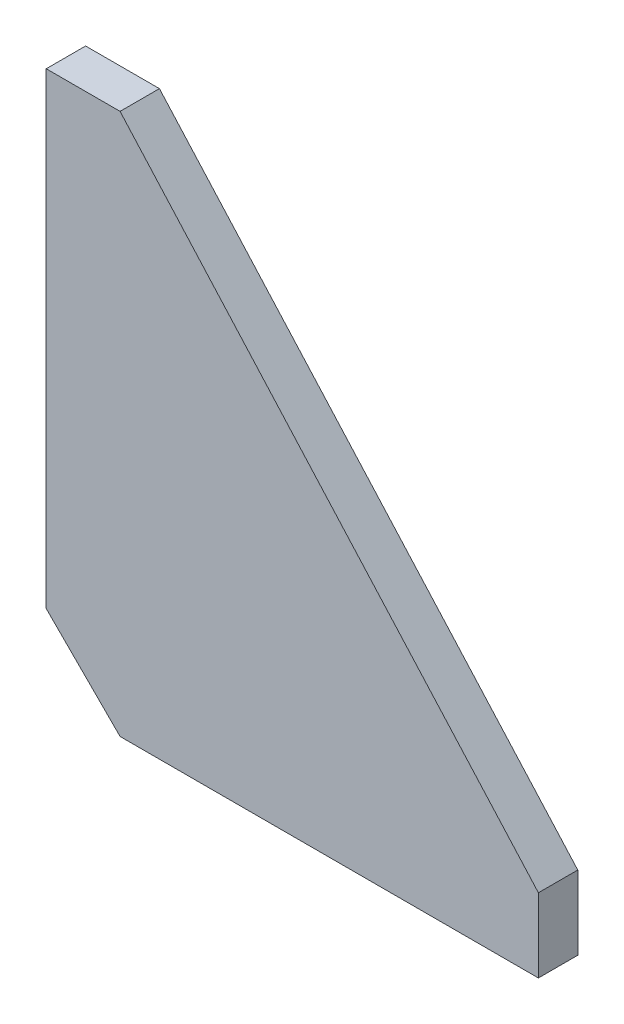
from build123d import *

# Parameters (mm, degrees)
EXTRUDE_1_DEPTH = 8
CHAMFER_1_SIZE  = 15


with BuildPart() as part:
    # 草图1 → 凸台-拉伸1 (new body)
    with BuildSketch(Plane.XY):
        Polygon((0, 0), (100, 0), (100, 15), (15, 110), (0, 110), align=None)
    extrude(amount=EXTRUDE_1_DEPTH)

    # 倒角1
    chamfer_1_edges = [part.edges().sort_by_distance(p)[0] for p in [
        (0, 0, 4),
    ]]
    chamfer(chamfer_1_edges, length=CHAMFER_1_SIZE)


solid = part.part
